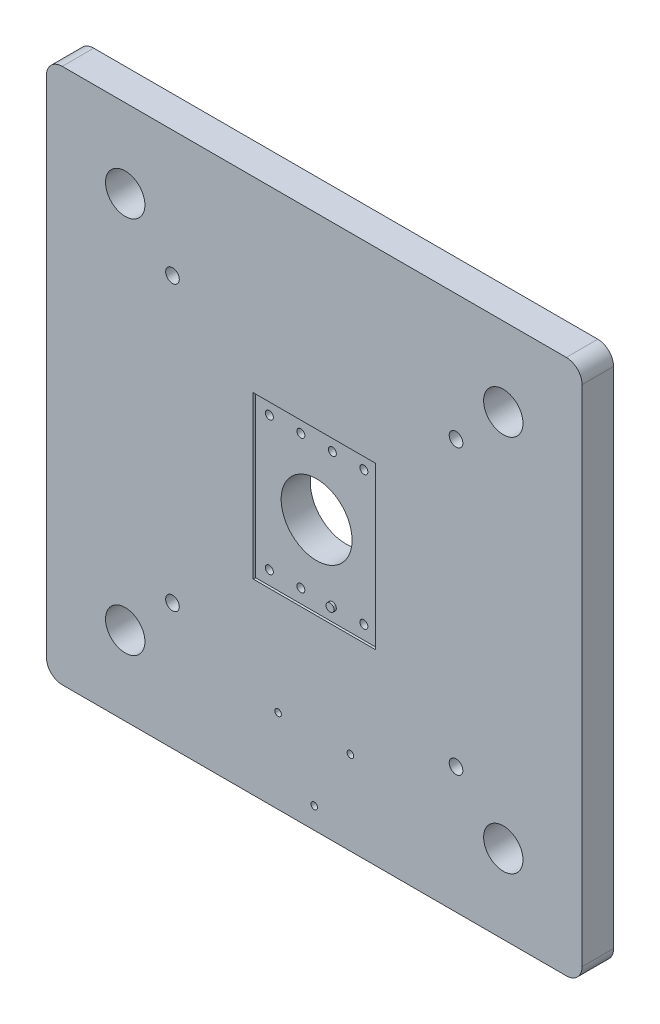
SolidWorks part; units mm, degrees
ref_plane "Front Plane" through (0, 0, 0) normal (0, 0, 1) x (1, 0, 0)
ref_plane "Top Plane" through (0, 0, 0) normal (0, 1, 0) x (1, 0, 0)
ref_plane "Right Plane" through (0, 0, 0) normal (1, 0, 0) x (0, 0, -1)
sketch "Sketch1" plane through (0, 0, 0) normal (0, 0, 1) x (1, 0, 0)
  line L1 (340, 340) -> (-340, 340)
  line L2 (340, 340) -> (340, -340)
  line L3 (340, -340) -> (-340, -340)
  line L4 (-340, 340) -> (-340, -340)
  line L5 (340, 340) -> (-340, -340) construction
  line L6 (340, -340) -> (-340, 340) construction
  point P0 (0, 0)
  dimension "D1" = 680
  dimension "D2" = 680
extrude "Boss-Extrude1" add sketch "Sketch1" along normal blind 40
fillet "Fillet1" radius 20 4 edges at (-340, -340, 20) (340, -340, 20) (-340, 340, 20) (340, 340, 20)
sketch "Sketch2" plane through (0, 0, 40) normal (0, 0, 1) x (1, 0, 0)
  line L0 (0, 0) -> (0, 62.2452) construction
  line L1 (77.5, 102.5) -> (-77.5, 102.5)
  line L2 (77.5, 102.5) -> (77.5, -102.5)
  line L3 (77.5, -102.5) -> (-77.5, -102.5)
  line L4 (-77.5, 102.5) -> (-77.5, -102.5)
  line L5 (77.5, 102.5) -> (-77.5, -102.5) construction
  line L6 (77.5, -102.5) -> (-77.5, 102.5) construction
  line L7 (0, 0) -> (32.4953, 0) construction
  circle A8 centre (-60, 85) radius 5.05
  circle A9 centre (-20, 85) radius 5.05
  circle A10 centre (20, 85) radius 5.05
  circle A11 centre (60, 85) radius 5.05
  circle A12 centre (60, -85) radius 5.05
  circle A13 centre (20, -85) radius 5.05
  circle A14 centre (-20, -85) radius 5.05
  circle A15 centre (-60, -85) radius 5.05
  point P0 (0, 0)
  dimension "D8" = 10.1
  dimension "D1" = 155
  dimension "D2" = 205
  dimension "D3" = 40
  dimension "D4" = 120
  dimension "D5" = 40
  dimension "D6" = 17.5
  dimension "D7" = 17.5
extrude "Cut-Extrude1" cut sketch "Sketch2" against normal blind 3
sketch "Sketch3" plane through (0, 0, 40) normal (0, 0, 1) x (1, 0, 0)
  circle A16 centre (-60, -85) radius 5.05 construction
  circle A17 centre (-60, 85) radius 5.05
  circle A18 centre (-60, 85) radius 5.05
  circle A19 centre (-20, -85) radius 5.05 construction
  circle A20 centre (60, -85) radius 5.05 construction
  circle A21 centre (60, 85) radius 5.05 construction
  circle A22 centre (20, 85) radius 5.05 construction
  circle A23 centre (-20, 85) radius 5.05 construction
  circle A24 centre (-60, -85) radius 5.05
  circle A25 centre (-20, -85) radius 5.05
  circle A26 centre (60, -85) radius 5.05
  circle A27 centre (60, 85) radius 5.05
  circle A28 centre (20, 85) radius 5.05
  circle A29 centre (-20, 85) radius 5.05
  dimension "D1" = 0
extrude "Cut-Extrude2" cut sketch "Sketch3" against normal blind 219
sketch "Sketch4" plane through (0, 0, 37) normal (0, 0, 1) x (1, 0, 0)
  circle A0 centre (0, 0) radius 45
  dimension "D1" = 90
extrude "Cut-Extrude3" cut sketch "Sketch4" against normal blind 219
sketch "Sketch5" plane through (0, 0, 40) normal (0, 0, 1) x (1, 0, 0)
  line L1 (180, 180) -> (-180, 180) construction
  line L2 (180, 180) -> (180, -180) construction
  line L3 (180, -180) -> (-180, -180) construction
  line L4 (-180, 180) -> (-180, -180) construction
  line L5 (180, 180) -> (-180, -180) construction
  line L6 (180, -180) -> (-180, 180) construction
  circle A0 centre (-180, 180) radius 8.65
  circle A1 centre (180, 180) radius 8.65
  circle A2 centre (180, -180) radius 8.65
  circle A3 centre (-180, -180) radius 8.65
  point P0 (0, 0)
  dimension "D3" = 17.3
  dimension "D1" = 360
  dimension "D2" = 360
extrude "Cut-Extrude4" cut sketch "Sketch5" against normal blind 219
sketch "Sketch6" plane through (0, 0, 40) normal (0, 0, 1) x (1, 0, 0)
  circle A3 centre (0, -313) radius 4.2
  circle A4 centre (45.8993, -233.5) radius 4.2
  circle A5 centre (-45.8993, -233.5) radius 4.2
  point P18 (0, 0)
extrude "Cut-Extrude5" cut sketch "Sketch6" against normal blind 219
sketch "Sketch7" plane through (0, 0, 40) normal (0, 0, 1) x (1, 0, 0)
  line L1 (240, 240) -> (-240, 240) construction
  line L2 (240, 240) -> (240, -240) construction
  line L3 (240, -240) -> (-240, -240) construction
  line L4 (-240, 240) -> (-240, -240) construction
  line L5 (240, 240) -> (-240, -240) construction
  line L6 (240, -240) -> (-240, 240) construction
  circle A0 centre (-240, 240) radius 25
  circle A1 centre (240, 240) radius 25
  circle A2 centre (240, -240) radius 25
  circle A3 centre (-240, -240) radius 25
  point P0 (0, 0)
  dimension "D3" = 50
  dimension "D1" = 480
  dimension "D2" = 480
extrude "Cut-Extrude6" cut sketch "Sketch7" against normal blind 219
